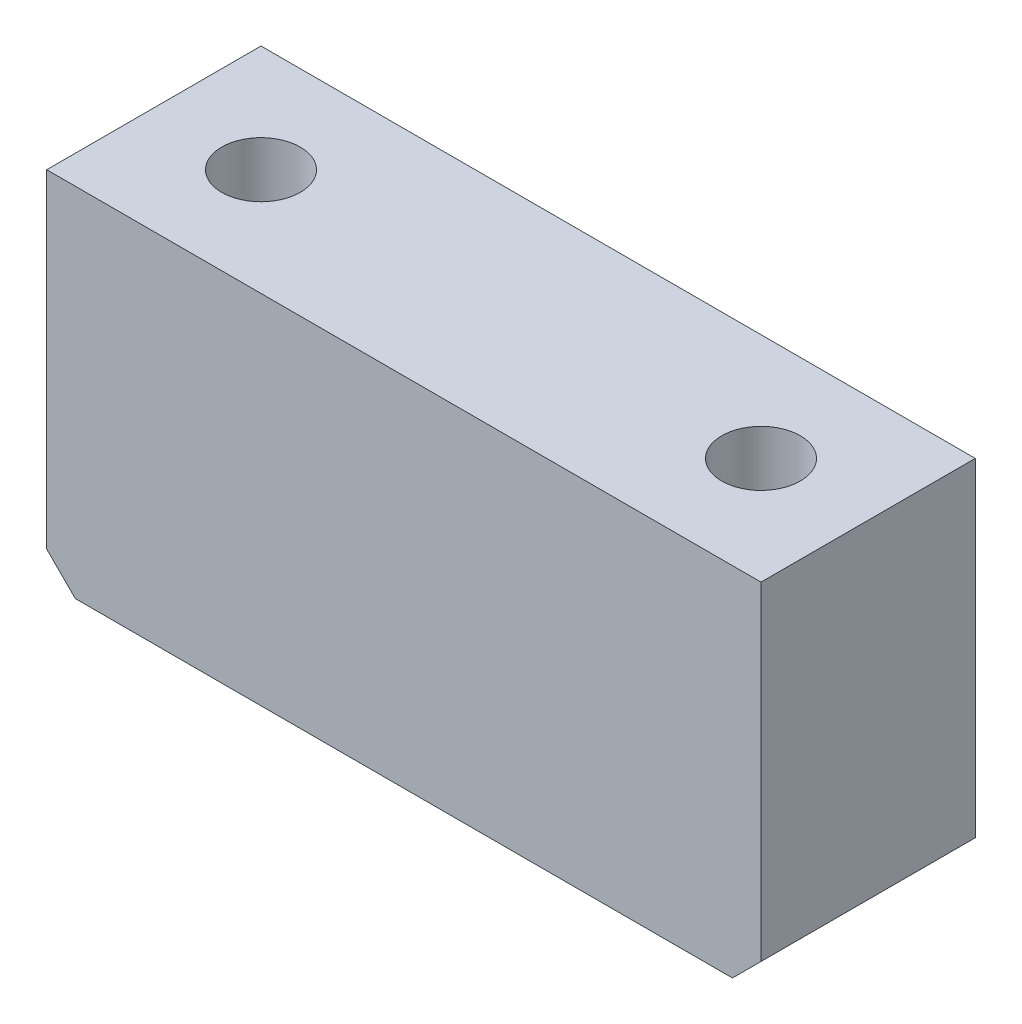
from build123d import *

# Parameters (mm, degrees)
SKETCH_1_W                   = 50
SKETCH_1_H                   = 25
EXTRUDE_1_DEPTH              = 15
CHAMFER_1_SIZE               = 2
HOLE_WIZARD_M5_1_D           = 5.5
HOLE_WIZARD_M5_1_CBORE_D     = 10
HOLE_WIZARD_M5_1_CBORE_DEPTH = 15.7


with BuildPart() as part:
    # 草图1 → 凸台-拉伸1 (new body)
    with BuildSketch(Plane.XY):
        Rectangle(SKETCH_1_W, SKETCH_1_H)
    extrude(amount=EXTRUDE_1_DEPTH)

    # 倒角1
    chamfer_1_edges = [part.edges().sort_by_distance(p)[0] for p in [
        (25, -12.5, 7.5),
        (-25, -12.5, 7.5),
    ]]
    chamfer(chamfer_1_edges, length=CHAMFER_1_SIZE)

    # M5 六角圆柱头螺钉的柱形沉头孔1 (through all)
    with Locations(Plane(origin=(0, -12.5, 0), x_dir=(-1, 0, 0), z_dir=(0, -1, 0))):
        with Locations((-17.5, -7.5), (17.5, -7.5)):
            CounterBoreHole(HOLE_WIZARD_M5_1_D / 2, HOLE_WIZARD_M5_1_CBORE_D / 2, HOLE_WIZARD_M5_1_CBORE_DEPTH)


solid = part.part
